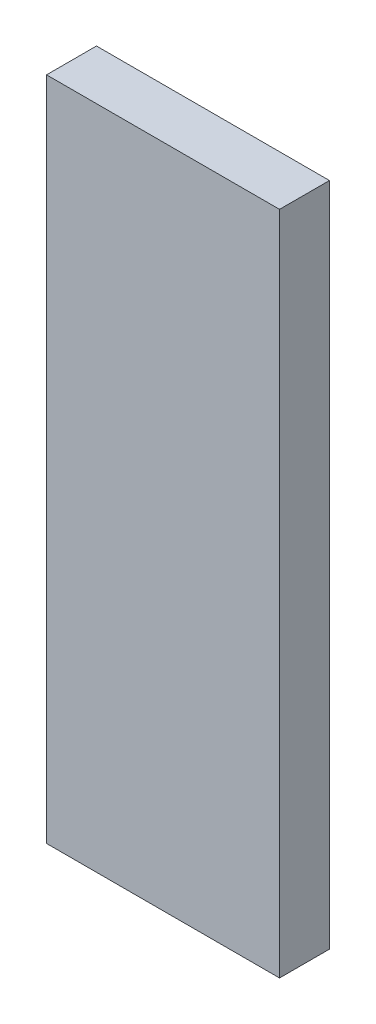
SolidWorks part; units mm, degrees
material "Q235-A"
ref_plane "Front Plane" through (0, 0, 0) normal (0, 0, 1) x (1, 0, 0)
ref_plane "Top Plane" through (0, 0, 0) normal (0, 1, 0) x (1, 0, 0)
ref_plane "Right Plane" through (0, 0, 0) normal (1, 0, 0) x (0, 0, -1)
sketch "Sketch1" plane through (0, 0, 0) normal (0, 0, 1) x (1, 0, 0)
  line L1 (35, -100) -> (-35, -100)
  line L2 (35, -100) -> (35, 100)
  line L3 (35, 100) -> (-35, 100)
  line L4 (-35, -100) -> (-35, 100)
  line L5 (35, -100) -> (-35, 100) construction
  line L6 (35, 100) -> (-35, -100) construction
  point P0 (0, 0)
  dimension "D1" = 70
  dimension "D2" = 200
extrude "Boss-Extrude1" add sketch "Sketch1" along normal mid plane 15
